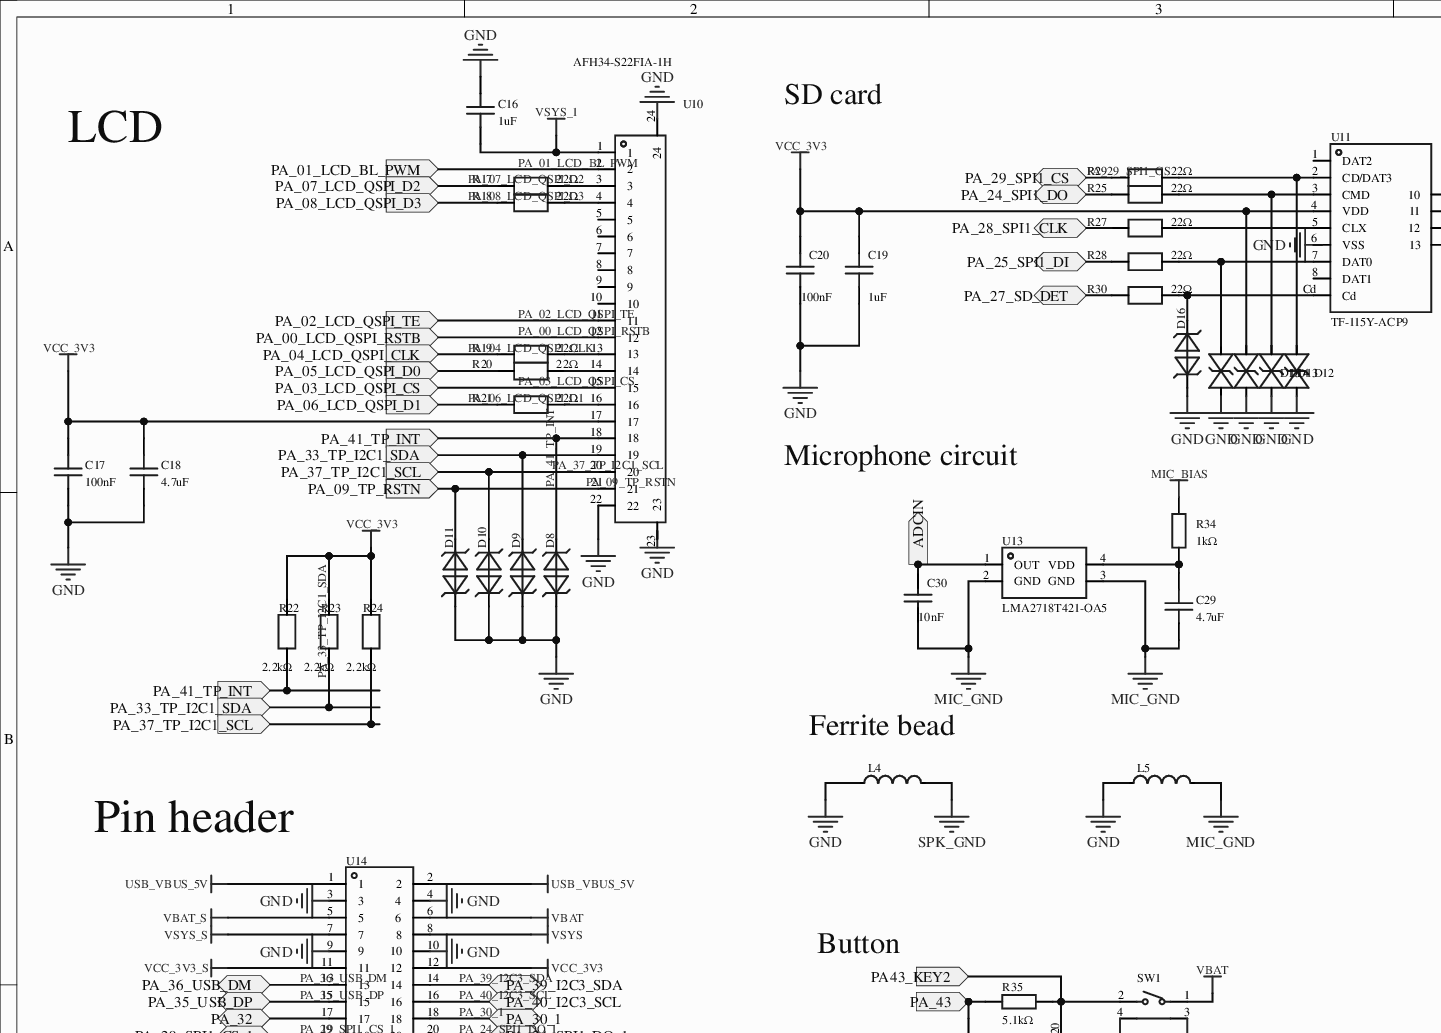
[diagram p0: MISC52032-4.schdoc, top left]
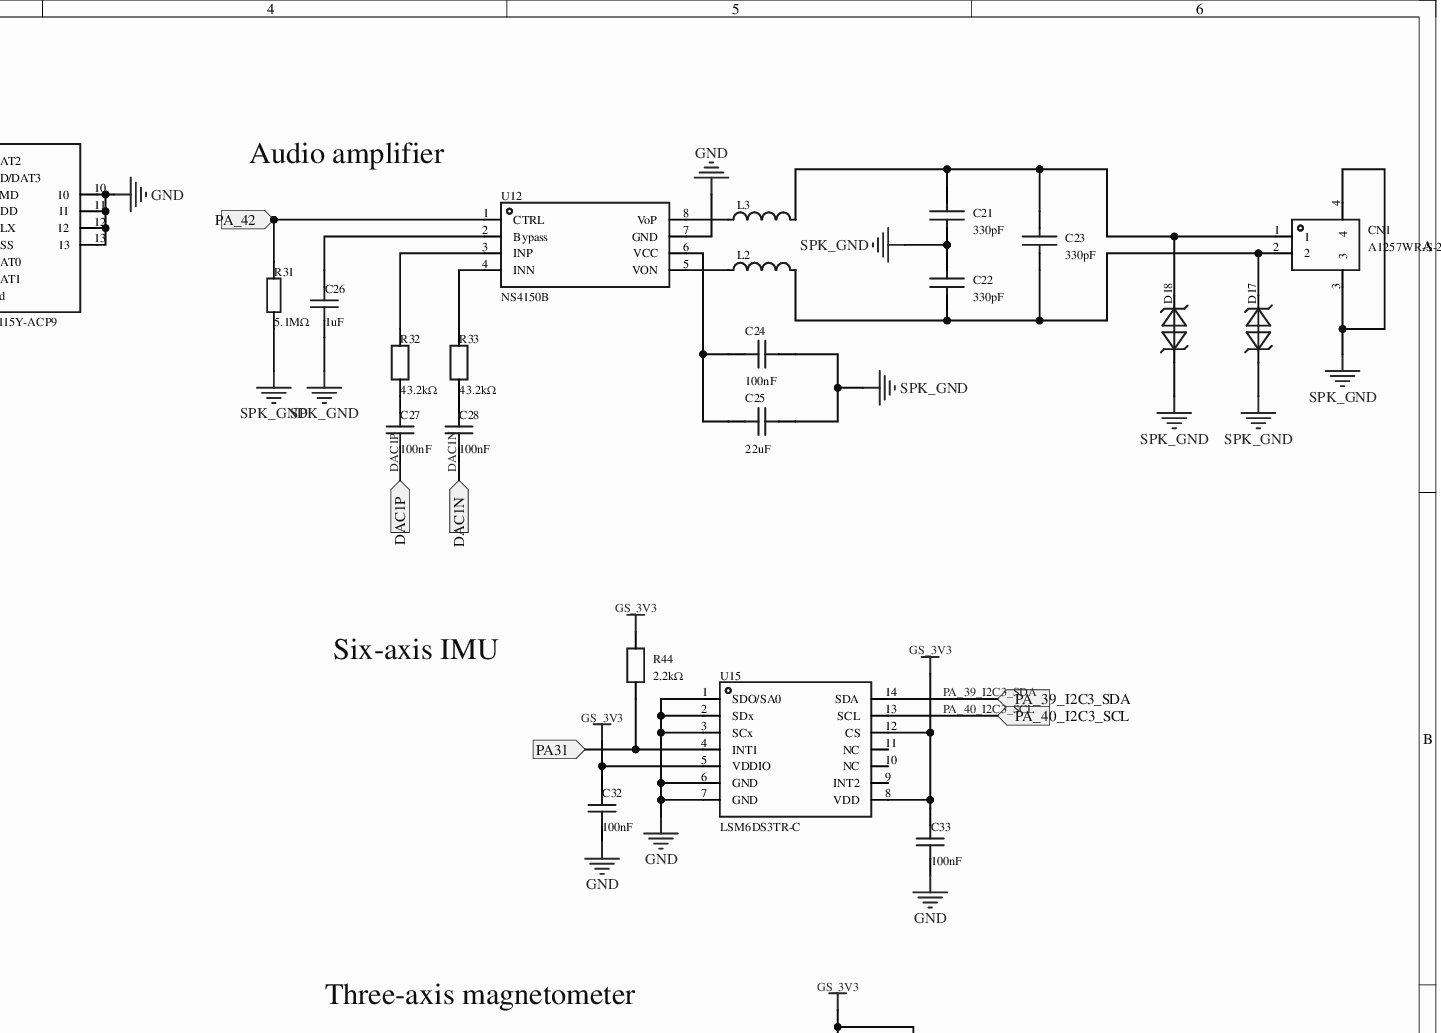
[diagram p1: MISC52032-4.schdoc, top right]
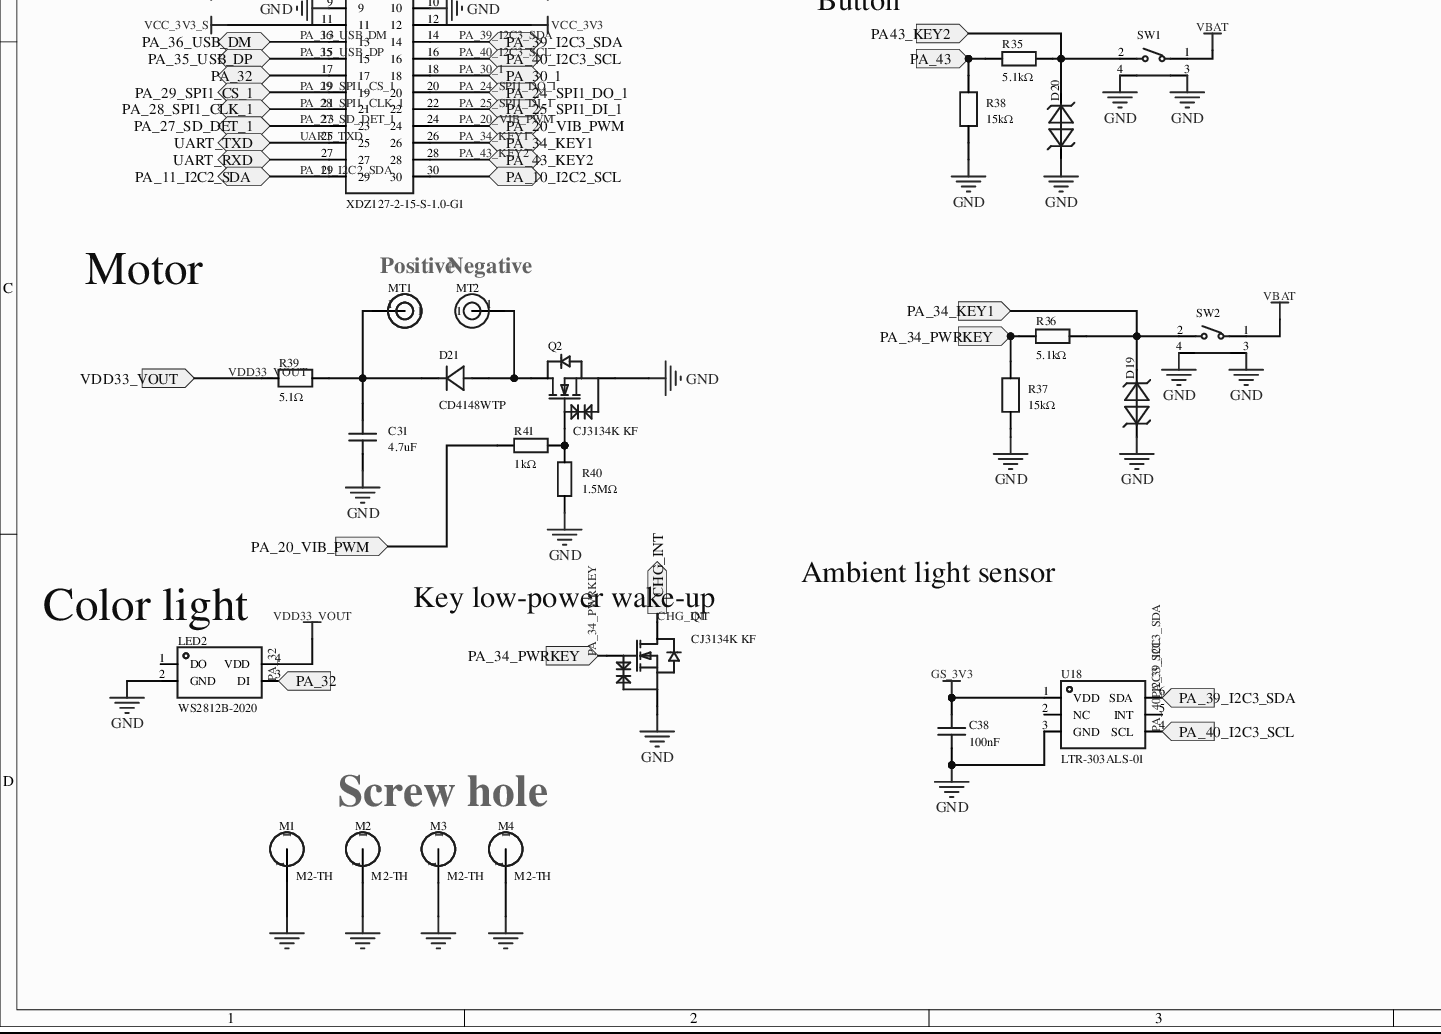
[diagram p2: MISC52032-4.schdoc, bottom left]
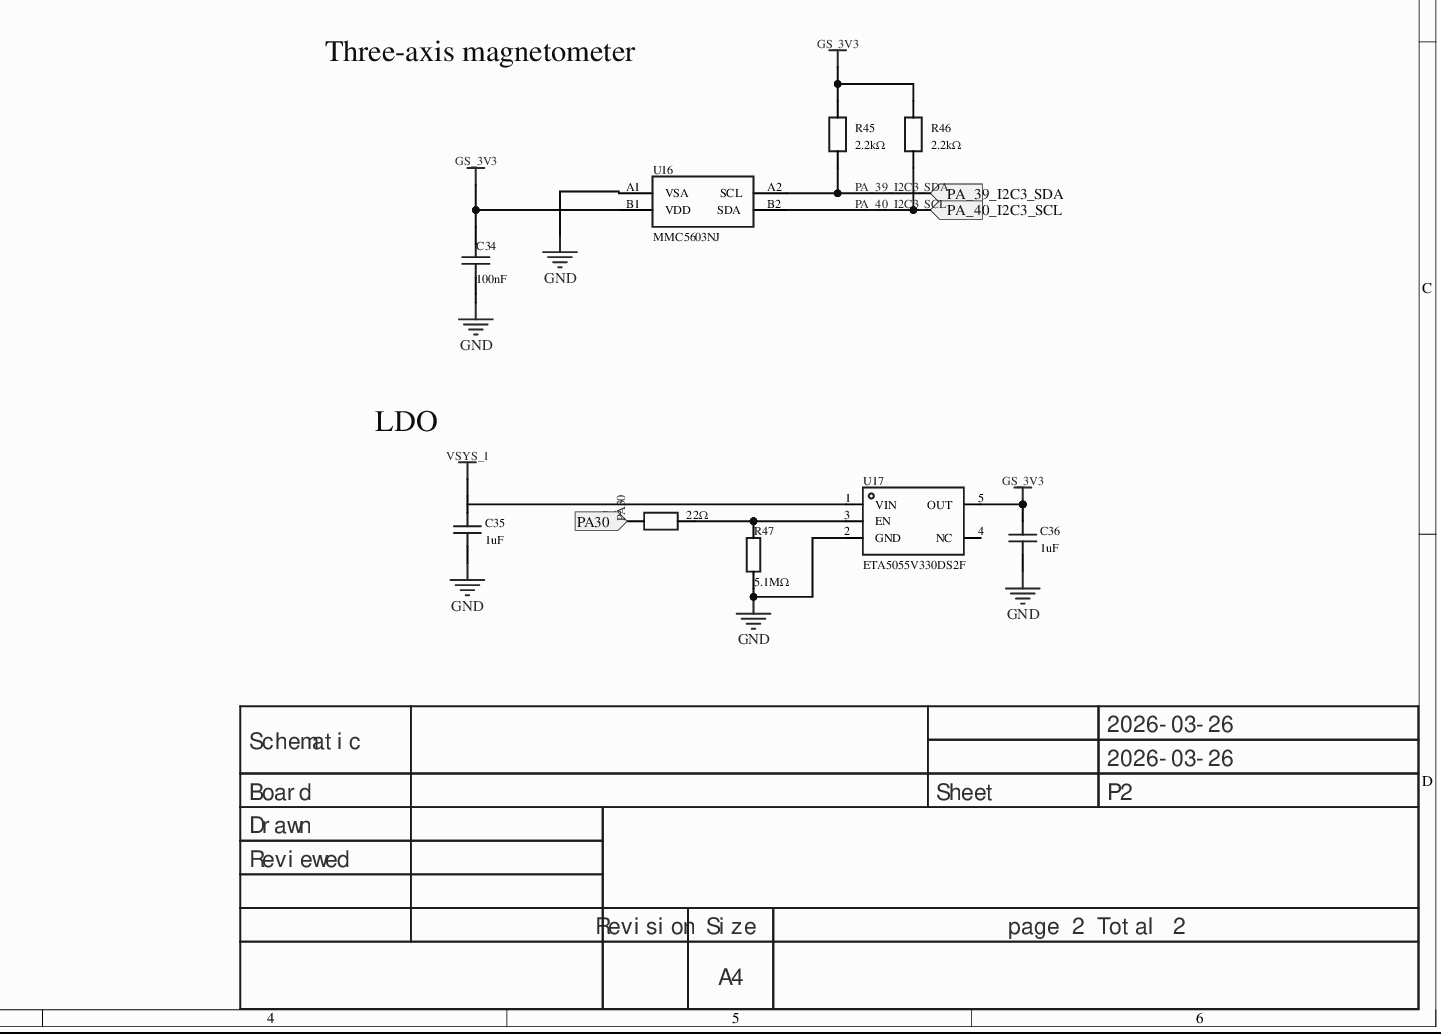
[diagram p3: MISC52032-4.schdoc, bottom right]
# Altium project MISC52032-2.PrjPcb (part 2 of 2)

## Sheet MISC52032-4.schdoc
size 420 x 297 mm; Version: V1.0; @Project Name: MISC52032; @Page Count: 2; @Update Date: 2026-03-26; @Create Date: 2026-03-26; @Schematic Name: MISC52032; @Page No: 2; @Board Name: MISC52032; @Create Time: 13:38:37; @Update Time: 21:26:46; Size: A4

### Parts
C16  1uF  [C0402]
C17  100nF  [C0402]
C18  4.7uF  [C0402]
C19  1uF  [C0402]
C20  100nF  [C0402]
C21  330pF  [C0402]
C22  330pF  [C0402]
C23  330pF  [C0402]
C24  100nF  [C0402]
C25  22uF  [C0402]
C26  1uF  [C0402]
C27  100nF  [C0402]
C28  100nF  [C0402]
C29  4.7uF  [C0402]
C30  10nF  [C0402]
C31  4.7uF  [C0402]
C32  100nF  [C0402]
C33  100nF  [C0402]
C34  100nF  [C0402]
C35  1uF  [C0402]
C36  1uF  [C0402]
C38  100nF  [C0402]
CN1  A1257WR-S-2P  [CONN-SMD_A1257WR-S-2P]
D8  ESD5451N  [DFN1006-2L-BI]  (value not drawn)
D9  ESD5451N  [DFN1006-2L-BI]  (value not drawn)
D10  ESD5451N  [DFN1006-2L-BI]  (value not drawn)
D11  ESD5451N  [DFN1006-2L-BI]  (value not drawn)
D12  (no value)  [D0402-BI]
D13  (no value)  [D0402-BI]
D14  (no value)  [D0402-BI]
D15  (no value)  [D0402-BI]
D16  ESD5451N  [DFN1006-2L-BI]  (value not drawn)
D17  ESD5451N  [DFN1006-2L-BI]  (value not drawn)
D18  ESD5451N  [DFN1006-2L-BI]  (value not drawn)
D19  ESD5451N  [DFN1006-2L-BI]  (value not drawn)
D20  ESD5451N  [DFN1006-2L-BI]  (value not drawn)
D21  CD4148WTP  [D0603-RD]
L2  (no value)  [L0402]
L3  (no value)  [L0402]
L4  (no value)  [L0603]
L5  (no value)  [L0603]
LED2  WS2812B-2020  [LED-SMD_4P-L2.0-W2.0-TL_WS2812B-2020]
M1  M2-TH  [M2_TH_4_2.5MM]
M2  M2-TH  [M2_TH_4_2.5MM]
M3  M2-TH  [M2_TH_4_2.5MM]
M4  M2-TH  [M2_TH_4_2.5MM]
MT1  (no value)  [TP-3x2MM]
MT2  (no value)  [TP-3x2MM]
Q1  CJ3134K KF  [SOT-723_L1.2-W0.8-P0.40-LS1.2-BR]
Q2  CJ3134K KF  [SOT-723_L1.2-W0.8-P0.40-LS1.2-BR]
R17  22Ω  [R0402]
R18  22Ω  [R0402]
R19  22Ω  [R0402]
R20  22Ω  [R0402]
R21  22Ω  [R0402]
R22  2.2kΩ  [R0402]
R23  2.2kΩ  [R0402]
R24  2.2kΩ  [R0402]
R25  22Ω  [R0402]
R27  22Ω  [R0402]
R28  22Ω  [R0402]
R29  22Ω  [R0402]
R30  22Ω  [R0402]
R31  5.1MΩ  [R0402]
R32  43.2kΩ  [R0402]
R33  43.2kΩ  [R0402]
R34  1kΩ  [R0402]
R35  5.1kΩ  [R0402]
R36  5.1kΩ  [R0402]
R37  15kΩ  [R0402]
R38  15kΩ  [R0402]
R39  5.1Ω  [R0402]
R40  1.5MΩ  [R0402]
R41  1kΩ  [R0402]
R44  2.2kΩ  [R0402]
R45  2.2kΩ  [R0402]
R46  2.2kΩ  [R0402]
R47  5.1MΩ  [R0402]
R48  22Ω  [R0402]
SW1  (no value)  [KEY-SMD_GT-TC191A-H026-L60]
SW2  (no value)  [KEY-SMD_GT-TC191A-H026-L60]
U10  AFH34-S22FIA-1H  [FPC-SMD_22P-P0.50_JS_AFH34-S22FIA-1H]
U11  TF-115Y-ACP9  [SIM-SMD_TF-115Y-BCP9]
U12  NS4150B  [MSOP-8_L3.0-W3.0-P0.65-LS5.0-BL]
U13  LMA2718T421-OA5  [MIC-SMD_4P-L2.8-W1.9-P1.01-TL]
U14  XDZ127-2-15-S-1.0-G1  [HDR-SMD_30P-P1.27-V-M-R2-C15-LS5.5_1]
U15  LSM6DS3TR-C  [LGA-14_L3.0-W2.5-P0.50-TL]
U16  MMC5603NJ  [FLIPCHIP-4_L0.8-W0.8-R2-C2-P0.40-TL]
U17  ETA5055V330DS2F  [SOT-23-5_L2.9-W1.6-P0.95-LS2.8-BR]
U18  LTR-303ALS-01  [TDFN-6_L2.0-W2.0-P0.65-BL]

### Ports
ADCIN (out), CHG_INT (out), DAC1N (in), DAC1P (in), PA30 (in), PA31 (in), PA43_KEY2 (in), PA_00_LCD_QSPI_RSTB (in), PA_01_LCD_BL_PWM (in), PA_02_LCD_QSPI_TE (in), PA_03_LCD_QSPI_CS (in), PA_04_LCD_QSPI_CLK (in), PA_05_LCD_QSPI_D0 (in), PA_06_LCD_QSPI_D1 (in), PA_07_LCD_QSPI_D2 (in), PA_08_LCD_QSPI_D3 (in), PA_09_TP_RSTN (in), PA_10_I2C2_SCL (bidir), PA_11_I2C2_SDA (bidir), PA_20_VIB_PWM (bidir), PA_20_VIB_PWM (in), PA_24_SPI1_DO (bidir), PA_24_SPI1_DO_1 (bidir), PA_25_SPI1_DI (bidir), PA_25_SPI1_DI_1 (bidir), PA_27_SD_DET (bidir), PA_27_SD_DET_1 (bidir), PA_28_SPI1_CLK (bidir), PA_28_SPI1_CLK_1 (bidir), PA_29_SPI1_CS (bidir), PA_29_SPI1_CS_1 (bidir), PA_30_1 (bidir), PA_32 (bidir), PA_32 (in), PA_33_TP_I2C1_SDA (in), PA_34_KEY1 (bidir), PA_34_KEY1 (in), PA_34_PWRKEY (in), PA_35_USB_DP (bidir), PA_36_USB_DM (bidir), PA_37_TP_I2C1_SCL (in), PA_39_I2C3_SDA (bidir), PA_39_I2C3_SDA (in), PA_40_I2C3_SCL (bidir), PA_40_I2C3_SCL (in), PA_41_TP_INT (in), PA_42 (in), PA_43 (in), PA_43_KEY2 (bidir), UART_RXD (bidir), UART_TXD (bidir), VDD33_VOUT (in)

### Nets
GND: C16.2 C17.1 C18.1 C19.1 C20.1 C31.1 C32.2 C33.2 C34.2 C35.1 C36.1 C38.1 D8.1 D9.1 D10.1 D11.1 D12.1(K) D13.1(K) D14.1(K) D15.1(K) D16.1 D19.1 D20.1 L4.1 L5.1 LED2.2(GND) M1.1 M2.1 M3.1 M4.1 Q1.2(S) Q2.2(S) R37.1 R38.1 R40.1 R47.1 SW1.3 SW1.4 SW2.3 SW2.4 U10.22 U10.23 U10.24 U11.6(VSS) U11.10 U11.11 U11.12 U11.13 U12.7(GND) U14.3 U14.4 U14.9 U14.10 U15.1(SDO/SA0) U15.2(SDx) U15.3(SCx) U15.6(GND) U15.7(GND) U16.A1(VSA) U17.2(GND) U18.3(GND)
GS_3V3: C32.1 C33.1 C34.1 C36.2 C38.2 R44.2 R45.2 R46.2 U15.5(VDDIO) U15.8(VDD) U15.12(CS) U16.B1(VDD) U17.5(OUT) U18.1(VDD)
MIC_BIAS: R34.2
MIC_GND: C29.1 C30.1 L5.2 U13.2(GND) U13.3(GND)
SPK_GND: C21.1 C22.2 C24.1 C25.1 C26.1 CN1.3 CN1.4 D17.1 D18.1 L4.2 R31.1
USB_VBUS_5V: U14.1 U14.2
VBAT: SW1.1 SW2.1 U14.6
VBAT_S: U14.5
VCC_3V3: C17.2 C18.2 C19.2 C20.2 D14.2(A) R22.2 R23.2 R24.2 U10.17 U11.4(VDD) U14.12
VCC_3V3_S: U14.11
VDD33_VOUT: LED2.4(VDD) R39.1 ; port VDD33_VOUT
VSYS: U14.8
VSYS_1: C16.1 C35.2 U10.1
VSYS_S: U14.7
ADCIN: C30.2 U13.1(OUT) ; port ADCIN
CHG_INT: Q1.3(D) ; port CHG_INT
DAC1N: C28.2 ; port DAC1N
DAC1P: C27.2 ; port DAC1P
PA30: R48.1 ; port PA30
PA_00_LCD_QSPI_RSTB: U10.12 ; port PA_00_LCD_QSPI_RSTB
PA_01_LCD_BL_PWM: U10.2 ; port PA_01_LCD_BL_PWM
PA_02_LCD_QSPI_TE: U10.11 ; port PA_02_LCD_QSPI_TE
PA_03_LCD_QSPI_CS: U10.15 ; port PA_03_LCD_QSPI_CS
PA_04_LCD_QSPI_CLK: R19.1 ; port PA_04_LCD_QSPI_CLK
PA_05_LCD_QSPI_D0: R20.1 ; port PA_05_LCD_QSPI_D0
PA_06_LCD_QSPI_D1: R21.1 ; port PA_06_LCD_QSPI_D1
PA_07_LCD_QSPI_D2: R17.1 ; port PA_07_LCD_QSPI_D2
PA_08_LCD_QSPI_D3: R18.1 ; port PA_08_LCD_QSPI_D3
PA_09_TP_RSTN: D11.2 U10.21 ; port PA_09_TP_RSTN
PA_10_I2C2_SCL: U14.30 ; port PA_10_I2C2_SCL
PA_11_I2C2_SDA: U14.29 ; port PA_11_I2C2_SDA
PA_20_VIB_PWM: R41.2 U14.24 ; port PA_20_VIB_PWM
PA_24_SPI1_DO_1: U14.20 ; port PA_24_SPI1_DO_1
PA_25_SPI1_DI: R28.1 ; port PA_25_SPI1_DI
PA_25_SPI1_DI_1: U14.22 ; port PA_25_SPI1_DI_1
PA_27_SD_DET: R30.1 ; port PA_27_SD_DET
PA_27_SD_DET_1: U14.23 ; port PA_27_SD_DET_1
PA_28_SPI1_CLK: R27.1 ; port PA_28_SPI1_CLK
PA_28_SPI1_CLK_1: U14.21 ; port PA_28_SPI1_CLK_1
PA_29_SPI1_CS: R29.1 ; port PA_29_SPI1_CS
PA_29_SPI1_CS_1: U14.19 ; port PA_29_SPI1_CS_1
PA_30_1: U14.18 ; port PA_30_1
PA_32: LED2.3(DI) U14.17 ; port PA_32
PA_33_TP_I2C1_SDA: D9.2 R23.1 U10.19 ; port PA_33_TP_I2C1_SDA
PA_34_KEY1: D19.2 R36.2 SW2.2 U14.26 ; port PA_34_KEY1
PA_34_PWRKEY: Q1.1(G) R36.1 R37.2 ; port PA_34_PWRKEY
PA_35_USB_DP: U14.15 ; port PA_35_USB_DP
PA_36_USB_DM: U14.13 ; port PA_36_USB_DM
PA_37_TP_I2C1_SCL: D10.2 R24.1 U10.20 ; port PA_37_TP_I2C1_SCL
PA_39_I2C3_SDA: R45.1 U14.14 U15.14(SDA) U16.A2(SCL) U18.6(SDA) ; port PA_39_I2C3_SDA
PA_40_I2C3_SCL: R46.1 U14.16 U15.13(SCL) U16.B2(SDA) U18.4(SCL) ; port PA_40_I2C3_SCL
PA_41_TP_INT: D8.2 R22.1 U10.18 ; port PA_41_TP_INT
PA_42: R31.2 U12.1(CTRL) ; port PA_42
PA_43: R35.1 R38.2 ; port PA_43
PA_43_KEY2: U14.28 ; port PA_43_KEY2
UART_RXD: U14.27 ; port UART_RXD
UART_TXD: U14.25 ; port UART_TXD
NetC21_2: C21.2 C23.2 CN1.1 D18.2 L3.2
NetC22_1: C22.1 C23.1 CN1.2 D17.2 L2.2
NetC24_2: C24.2 C25.2 U12.6(VCC)
NetC26_2: C26.2 U12.2(Bypass)
NetC27_1: C27.1 R32.1
NetC28_1: C28.1 R33.1
NetC29_2: C29.2 R34.1 U13.4(VDD)
NetC31_2: C31.2 D21.1(K) MT1.1 R39.2
NetD12_2: D12.2(A) R29.2 U11.2(CD/DAT3)
NetD13_2: D13.2(A) R25.2 U11.3(CMD)
NetD15_2: D15.2(A) R28.2 U11.7(DAT0)
NetD16_2: D16.2 R30.2 U11.Cd
NetD20_2: D20.2 R35.2 SW1.2 ; port PA43_KEY2
NetD21_2: D21.2(A) MT2.1 Q2.3(D)
NetL2_1: L2.1 U12.5(VON)
NetL3_1: L3.1 U12.8(VoP)
NetQ2_1: Q2.1(G) R40.2 R41.1
NetR17_2: R17.2 U10.3
NetR18_2: R18.2 U10.4
NetR19_2: R19.2 U10.13
NetR20_2: R20.2 U10.14
NetR21_2: R21.2 U10.16
NetR25_1: R25.1 ; port PA_24_SPI1_DO
NetR27_2: R27.2 U11.5(CLX)
NetR32_2: R32.2 U12.3(INP)
NetR33_2: R33.2 U12.4(INN)
NetR44_1: R44.1 U15.4(INT1) ; port PA31
NetR47_2: R47.2 R48.2 U17.3(EN)

Not connected (* = marked no-connect by the designer): LED2 1(DO)*; U10 5* 6* 7* 8* 9* 10*; U11 1(DAT2)* 8(DAT1)*; U15 9(INT2)* 10(NC)* 11(NC)*; U17 1(VIN) 4(NC)*; U18 2(NC)* 5(INT)*

### Notes on the sheet
- LCD
- SD card
- (near U12) Audio amplifier
- Microphone circuit
- Six-axis IMU
- (near L4) Ferrite bead
- (near U14) Pin header
- Button
- Three-axis magnetometer
- Motor
- Positive
- Negative
- LDO
- (near LED2) Color light
- (near Q1) Key low-power wake-up
- Ambient light sensor
- Screw hole
- 2026-03-26
- Schematic
- Board
- Sheet
- P2
- Drawn
- Reviewed
- Revision
- Size
- A4
- page 2 Total 2

### Library data of the parts
C16 C19 C26 C35 C36 = CL05A105KA5NQNC: Capacitance:1uF;Tolerance:±10%;Rated voltage:25V;Temperature coefficient:X5R;; Manufacturer: SAMSUNG(三星); AddInBom: yes; ModelId: 36a51122f27c49738f86b3bfa98863e0; ModelName: C0402_L1.0-W0.5-H0.5; ModelTransform: 39.37,19.685,0,0,0,0,0,0,0; Tolerance: ±10%; Voltage Rating: 25V; Temperature Coefficient: X5R; Symbol: CL05A105KA5NQNC; Device: CL05A105KA5NQNC; LCSC Part Name: 1uF ±10% 25V; SupplierPart: C52923; ManufacturerPart: CL05A105KA5NQNC; Supplier Footprint: 0402; JLCPCB Part Class: Basic library; Datasheet: example.com/datasheet/CL05A105KA5NQNC/53938.html; Supplier: LCSC; ConvertToPcb: yes; FootprintName: C0402; Value: 1uF
C17 C20 C24 C27 C28 C32-C34 C38 = CL05B104KO5NNNC: Capacitance:100nF;Tolerance:±10%;Rated voltage:16V;Temperature coefficient:X7R;; Manufacturer: SAMSUNG(三星); AddInBom: yes; ModelId: 36a51122f27c49738f86b3bfa98863e0; ModelName: C0402_L1.0-W0.5-H0.5; ModelTransform: 39.37,19.685,0,0,0,0,0,0,0; Tolerance: ±10%; Voltage Rating: 16V; Temperature Coefficient: X7R; Symbol: CL05B104KO5NNNC; Device: CL05B104KO5NNNC; LCSC Part Name: 100nF ±10% 16V; SupplierPart: C1525; ManufacturerPart: CL05B104KO5NNNC; Supplier Footprint: 0402; JLCPCB Part Class: Basic library; Datasheet: example.com/datasheet/CL05B104KO5NNNC/1877.html; Supplier: LCSC; ConvertToPcb: yes; FootprintName: C0402; Value: 100nF
C18 C29 C31 = CL05A475MP5NRNC: Capacitance:4.7uF;Tolerance:±20%;Rated voltage:10V;Temperature coefficient:X5R;; Manufacturer: SAMSUNG(三星); AddInBom: yes; ModelId: 36a51122f27c49738f86b3bfa98863e0; ModelName: C0402_L1.0-W0.5-H0.5; ModelTransform: 39.37,19.685,0,0,0,0,0,0,0; Tolerance: ±20%; Voltage Rating: 10V; Temperature Coefficient: X5R; Symbol: CL05A475MP5NRNC; Device: CL05A475MP5NRNC; LCSC Part Name: 4.7uF ±20% 10V; SupplierPart: C23733; ManufacturerPart: CL05A475MP5NRNC; Supplier Footprint: 0402; JLCPCB Part Class: Basic library; Datasheet: example.com/datasheet/CL05A475MP5NRNC/24469.html; Supplier: LCSC; ConvertToPcb: yes; FootprintName: C0402; Value: 4.7uF
C21-C23 = CL05C331JB5NNNC: Capacitance:330pF;Tolerance:±5%;Rated voltage:50V;Temperature coefficient:C0G;; Manufacturer: SAMSUNG(三星); AddInBom: yes; ModelId: 36a51122f27c49738f86b3bfa98863e0; ModelName: C0402_L1.0-W0.5-H0.5; ModelTransform: 39.37,19.685,0,0,0,0,0,0,0; Tolerance: ±5%; Voltage Rating: 50V; Temperature Coefficient: C0G; Symbol: CL05C331JB5NNNC; Device: CL05C331JB5NNNC; LCSC Part Name: 330pF ±5% 50V; SupplierPart: C13533; ManufacturerPart: CL05C331JB5NNNC; Supplier Footprint: 0402; JLCPCB Part Class: Extended library; Datasheet: example.com/datasheet/CL05C331JB5NNNC/14182.html; Supplier: LCSC; ConvertToPcb: yes; FootprintName: C0402; Value: 330pF
C25 = GRM155R60J226ME11D: Capacitance:22uF;Tolerance:±20%;Rated voltage:6.3V;Temperature coefficient:X5R;; Manufacturer: muRata(村田); AddInBom: yes; ModelId: 36a51122f27c49738f86b3bfa98863e0; ModelName: C0402_L1.0-W0.5-H0.5; ModelTransform: 39.37,19.685,0,0,0,0,0,0,0; Tolerance: ±20%; Voltage Rating: 6.3V; Temperature Coefficient: X5R; Symbol: GRM155R60J226ME11D; Device: GRM155R60J226ME11D; LCSC Part Name: 22uF ±20% 6.3V; SupplierPart: C415703; ManufacturerPart: GRM155R60J226ME11D; Supplier Footprint: 0402; JLCPCB Part Class: Extended library; Datasheet: example.com/datasheet/GRM155R60J226ME11D/408393.html; Supplier: LCSC; ConvertToPcb: yes; FootprintName: C0402; Value: 22uF
C30 = CL05B103KB5NNNC: Capacitance:10nF;Tolerance:±10%;Rated voltage:50V;Temperature coefficient:X7R;; Manufacturer: SAMSUNG(三星); AddInBom: yes; ModelId: 36a51122f27c49738f86b3bfa98863e0; ModelName: C0402_L1.0-W0.5-H0.5; ModelTransform: 39.37,19.685,0,0,0,0,0,0,0; Tolerance: ±10%; Voltage Rating: 50V; Temperature Coefficient: X7R; Symbol: CL05B103KB5NNNC; Device: CL05B103KB5NNNC; LCSC Part Name: 10nF ±10% 50V; SupplierPart: C15195; ManufacturerPart: CL05B103KB5NNNC; Supplier Footprint: 0402; JLCPCB Part Class: Basic library; Datasheet: example.com/datasheet/CL05B103KB5NNNC/15869.html; Supplier: LCSC; ConvertToPcb: yes; FootprintName: C0402; Value: 10nF
CN1 = A1257WR-S-2P: Pin structure:1x2P;Pitch:1.25mm;Mounting:Horizontal;Reference series:GH;Total pins:2P;Rows:1;Pins per row:2;Row spacing:-;Rated current:1A;Contact material:Phosphor bronze;Contact plating:Tin;Operating temperature:-40℃~+105℃;; Manufacturer: CJT(长江连接器); AddInBom: yes; ModelId: dbecf4c343244a1e903fd8658ee1ce26; ModelName: CONN-SMD_GH1.25-WS-2P; ModelTransform: 226.378,191.3382,0,0,0,0,0,-16.811,0; Pins Structure: 1x2P; Pitch: 1.25mm; Reference Series: GH; Number of PINs Per Row: 2; Current Rating: 1A; Voltage Rating: 50V; Plastic Material: PA9T; Flame Retardant Rating: UL94V-0; Symbol: A1257WR-S-2P; Device: A1257WR-S-2P; LCSC Part Name: 1x2P 间距:1.25mm 卧贴 系列:GH; SupplierPart: C225125; ManufacturerPart: A1257WR-S-2P; Supplier Footprint: SMD,P=1.25mm,卧贴; JLCPCB Part Class: Extended library; Datasheet: example.com/datasheet/A1257WR-S-2P/225408.html; Supplier: LCSC; ConvertToPcb: yes; FootprintName: CONN-SMD_A1257WR-S-2P; Mounting Type: Horizontal mount; Number of Pins: 2P; Number of Rows: 1; Row Spacing: -; Contact Material: Phosphor bronze; Contact Plating: Tin; Operating Temperature: -40℃~+105℃; Color: -
D8-D11 D16-D20 = ESD5451N: Manufacturer: UMW(友台半导体); 3D Model: 2bdbcca3b35b49c5a8ae725a08658930; Type: ESD; AddInBom: yes; ModelTransform: 40.1574,24.4094,0,0,0,0,0,0,0; Supplier Footprint: DFN1006-2; JLCPCB Part Class: Extended Part; Datasheet: example.com/upload/public/pdf/source/20231109/ADF50DFDA976AEDE26D2560D9AE1EB02.pdf; Device: ESD5451N; Symbol: ESD5451N; LCSC Part Name: ESD5451N; SupplierPart: C2987696; ManufacturerPart: ESD5451N; Supplier: LCSC; ConvertToPcb: yes; FootprintName: DFN1006-2L-BI; ModelName: DFN1006-2L-BI
D12-D15 = KLXES15AAA1: Polarity:Bidirectional;Reverse standoff voltage (Vrwm):5V;Clamping voltage:40V;Peak pulse current (Ipp):-;Peak pulse power (Ppp):-;Breakdown voltage:-;; Manufacturer: KUU; AddInBom: yes; ModelId: 62a80a189f1b46df8ba79817b730b378; ModelName: D0402_L1.0-W0.5-H0.5; ModelTransform: 39.37,19.685,0,0,0,0,0,0,0; Reverse Stand-Off Voltage (Vrwm): 5V; Clamping Voltage: 40V; Reverse Leakage Current (Ir): 10nA; Number of Channels: Single channel; level of protection: IEC 61000-4-2; Type: ESD; Junction Capacitance: 0.05pF; Symbol: KLXES15AAA1; Device: KLXES15AAA1; LCSC Part Name: 双向ESD 5V截止; SupplierPart: C2892490; Supplier Footprint: 0402; JLCPCB Part Class: Extended library; Datasheet: example.com/datasheet/KLXES15AAA1/3124109.html; Supplier: LCSC; ConvertToPcb: yes; FootprintName: D0402-BI; Polarity: Bidirectional; Peak Pulse Current (Ipp): -; Peak Pulse Power Dissipation (Ppp): -; Voltage - Breakdown: -; Operating Temperature: -55℃~+125℃
D21 = CD4148WTP_C30584800: Diode configuration:Discrete;Forward voltage (Vf):1.25V@100mA;DC reverse voltage (Vr):75V;Rectified current:150mA;Reverse recovery time (Trr):4ns;; Manufacturer: YONGYUTAI(永裕泰); AddInBom: yes; ModelId: 35f9a12e738d4b13b3012a5e6f6e8360; ModelTransform: 61.024,31.496,0,0,0,0,0,0,0; Voltage - DC Reverse(Vr): 75V; Current - Rectified: 150mA; Pd - Power Dissipation: 200mW; Reverse Leakage Current (Ir): 5uA@75V; Reverse Recovery Time (trr): 4ns; Operating Junction Temperature Range: -55℃~+150℃@(Tj); Non-Repetitive Peak Forward Surge Current: 800mA; Symbol: CD4148WTP_C30584800; Device: CD4148WTP_C30584800; LCSC Part Name: 75V 150mA; SupplierPart: C30584800; ManufacturerPart: CD4148WTP; Supplier Footprint: 0603; JLCPCB Part Class: Extended library; Datasheet: example.com/datasheet/CD4148WTP/32319012.html; Supplier: LCSC; ConvertToPcb: yes; FootprintName: D0603-RD; ModelName: D0603-RD; Diode Configuration: Discrete; Voltage - Forward(Vf@If): 1.25V@100mA
L2 L3 = PZ1005U121-1R0TF: Impedance@frequency:120Ω@100MHz;Tolerance:±25%;DC resistance (DCR):120mΩ;; Manufacturer: Sunlord(顺络); AddInBom: yes; ModelId: d8d36575a3234d4790bfa765c88664a7; ModelName: L0402_L1.0-W0.5-H0.5_BEAD; ModelTransform: 39.37,19.685,0,0,0,0,0,0.0005,0; Tolerance: ±25%; DC Resistance(DCR): 120mΩ; Current Rating: 1A; Number of Circuits: 1; Symbol: PZ1005U121-1R0TF; Device: PZ1005U121-1R0TF; LCSC Part Name: 单路 0402磁珠 阻抗120Ω@100MHz; SupplierPart: C96723; Supplier Footprint: 0402; JLCPCB Part Class: Extended library; Datasheet: example.com/datasheet/PZ1005U121-1R0TF/97928.html; Supplier: LCSC; ConvertToPcb: yes; FootprintName: L0402; Impedance @ Frequency: 120Ω@100MHz
L4 L5 = CBG160808U000T: Impedance@frequency:0Ω@100MHz;DC resistance (DCR):100mΩ;; Manufacturer: FH(风华); AddInBom: yes; ModelId: 2bc5ec593d464d6ba9807aec0b5673c2; ModelName: L0603_L1.6-W0.8-H0.5_BEAD; ModelTransform: 62.992,31.496,0,180,0,0,0.094,0.629,0; DC Resistance(DCR): 100mΩ; Current Rating: 800mA; Number of Circuits: 1; Symbol: CBG160808U000T; Device: CBG160808U000T; LCSC Part Name: 单路 0603磁珠 阻抗0Ω@100MHz; SupplierPart: C43163; Supplier Footprint: 0603; JLCPCB Part Class: Extended library; Datasheet: example.com/datasheet/CBG160808U000T/44154.html; Supplier: LCSC; ConvertToPcb: yes; FootprintName: L0603; Impedance @ Frequency: 0Ω@100MHz; Operating Temperature: -40℃~+85℃
LED2 = WS2812B-2020: 12mA, small size, high brightness, for small-pitch small-size products (note moisture sensitivity; see datasheet for details); Manufacturer: worldsemi; AddInBom: yes; ModelId: ec3f1773c2c342958c28fcec35b8a247; ModelName: LED-SMD_4P-L2.0-W2.0-H0.8-TL_WS2812B-2020; ModelTransform: 78.74,78.74,0,0,0,0,0.001,0.005,0; Wavelength: 515.6nm; 622.5nm; 470.4nm; Luminous Intensity: 200mcd; 160mcd; 520mcd; Data Transmission Rate: 100KB/S; Voltage - Supply: 5V; Installation method: Top mount; Symbol: WS2812B-2020; Device: WS2812B-2020; LCSC Part Name: RGB三色; SupplierPart: C965555; ManufacturerPart: WS2812B-2020; Supplier Footprint: SMD,2.2x2mm; JLCPCB Part Class: Extended library; Datasheet: example.com/datasheet/WS2812B-2020/1051115.html; Supplier: LCSC; ConvertToPcb: yes; FootprintName: LED-SMD_4P-L2.0-W2.0-TL_WS2812B-2020; Fixed-Frequency Pwm Mode: -; Quiescent Current: -; Lens Color: -; ESD Withstand Voltage: -; Operating Temperature: -
M1-M4 = M2-TH: Check: false; AddInBom: no; ConvertToPcb: yes; Device: M2-TH; SymbolName: M2-TH; FootprintName: M2_TH_4_2.5MM; Value: M2-TH
MT1 MT2 = TP_2x3MM: Add into BOM: no; Check: false; ConvertToPcb: yes; SymbolName: TP; Device: TP_2x3MM; FootprintName: TP-3x2MM
Q1 Q2 = CJ3134K KF: Type:1 N-channel;Drain-source voltage (Vdss):20V;Continuous drain current (Id):750mA;On-resistance (RDS(on)):380mΩ@4.5V,650mA;Power dissipation (Pd):150mW;Threshold voltage (Vgs(th)):1.1V;; Manufacturer: CJ(江苏长电/长晶); Symbol: CJ3134K_C62503; AddInBom: yes; ModelId: abccde1e67074d7481274a37cf5c97f0; ModelName: SOT-723-3P_L1.2-W0.8-H0.6-LS1.2-P0.40; ModelTransform: 47.244,47.244,0,180,0,0,0,0,0; Drain to Source Voltage: 20V; Current - Continuous Drain(Id): 750mA; Pd - Power Dissipation: 150mW; Gate Threshold Voltage (Vgs(th)@Id): 1.1V; Device: CJ3134K KF; LCSC Part Name: 1个N沟道 耐压:20V 电流:750mA; SupplierPart: C62503; ManufacturerPart: CJ3134K KF; Supplier Footprint: SOT-723; JLCPCB Part Class: Extended library; Datasheet: example.com/upload/public/pdf/source/20160416/1460799387864.pdf; Supplier: LCSC; ConvertToPcb: yes; FootprintName: SOT-723_L1.2-W0.8-P0.40-LS1.2-BR; Type: 1 N-channel; RDS(on): 380mΩ@4.5V,650mA
R17-R21 R25 R27-R30 R48 = FRC0402J220 TS: Resistor type:Thick-film resistor;Resistance:22Ω;Tolerance:±5%;Power:62.5mW;Operating voltage:50V;Temperature coefficient:±100ppm/℃;; Manufacturer: FOJAN(富捷); AddInBom: yes; ModelId: 98c88bc2b9094f218f3a3e30a7012738; ModelName: R0402_L1.0-W0.5-H0.4; ModelTransform: 39.37,19.685,0,0,0,0,0,0,0; Tolerance: ±5%; Power(Watts): 62.5mW; Voltage-Supply(Max): 50V; Symbol: FRC0402J220 TS; Device: FRC0402J220 TS; LCSC Part Name: 22Ω ±5% 62.5mW 厚膜电阻; SupplierPart: C2906914; ManufacturerPart: FRC0402J220 TS; Supplier Footprint: 0402; JLCPCB Part Class: Extended library; Datasheet: example.com/datasheet/FRC0402J220%2520TS/3180427.html; Supplier: LCSC; ConvertToPcb: yes; FootprintName: R0402; Type: Thick-film resistor; Value: 22Ω; Temperature Coefficient: ±100ppm/℃; Operating Temperature: -55℃~+155℃
R22-R24 R44-R46 = FRC0402F2201TS: Resistor type:Thick-film resistor;Resistance:2.2kΩ;Tolerance:±1%;Power:62.5mW;Operating voltage:50V;Temperature coefficient:±100ppm/℃;; Manufacturer: FOJAN(富捷); AddInBom: yes; ModelId: 98c88bc2b9094f218f3a3e30a7012738; ModelName: R0402_L1.0-W0.5-H0.4; ModelTransform: 39.37,19.685,0,0,0,0,0,0,0; Tolerance: ±1%; Power(Watts): 62.5mW; Voltage-Supply(Max): 50V; Symbol: FRC0402F2201TS; Device: FRC0402F2201TS; LCSC Part Name: 2.2kΩ ±1% 62.5mW 厚膜电阻; SupplierPart: C2906865; ManufacturerPart: FRC0402F2201TS; Supplier Footprint: 0402; JLCPCB Part Class: Extended library; Datasheet: example.com/datasheet/FRC0402F2201TS/3180378.html; Supplier: LCSC; ConvertToPcb: yes; FootprintName: R0402; Type: Thick-film resistor; Value: 2.2kΩ; Temperature Coefficient: ±100ppm/℃; Operating Temperature: -55℃~+155℃
R31 R47 = 0402WGF5104TCE: Resistor type:Thick-film resistor;Resistance:5.1MΩ;Tolerance:±1%;Power:62.5mW;Operating voltage:50V;Temperature coefficient:±100ppm/℃;; Manufacturer: UNI-ROYAL(厚声); AddInBom: yes; ModelId: 98c88bc2b9094f218f3a3e30a7012738; ModelName: R0402_L1.0-W0.5-H0.4; ModelTransform: 39.37,19.685,0,0,0,0,0,0,0; Tolerance: ±1%; Power(Watts): 62.5mW; Voltage-Supply(Max): 50V; Symbol: 0402WGF5104TCE; Device: 0402WGF5104TCE; LCSC Part Name: 5.1MΩ ±1% 62.5mW 厚膜电阻; SupplierPart: C270595; ManufacturerPart: 0402WGF5104TCE; Supplier Footprint: 0402; JLCPCB Part Class: Extended library; Datasheet: example.com/datasheet/0402WGF5104TCE/259975.html; Supplier: LCSC; ConvertToPcb: yes; FootprintName: R0402; Type: Thick-film resistor; Value: 5.1MΩ; Temperature Coefficient: ±100ppm/℃; Operating Temperature: -55℃~+155℃
R32 R33 = FRC0402F4322TS: Resistor type:Thick-film resistor;Resistance:43.2kΩ;Tolerance:±1%;Power:62.5mW;Operating voltage:50V;Temperature coefficient:±100ppm/℃;; Manufacturer: FOJAN(富捷); AddInBom: yes; ModelId: 98c88bc2b9094f218f3a3e30a7012738; ModelName: R0402_L1.0-W0.5-H0.4; ModelTransform: 39.37,19.685,0,0,0,0,0,0,0; Tolerance: ±1%; Power(Watts): 62.5mW; Voltage-Supply(Max): 50V; Symbol: FRC0402F4322TS; Device: FRC0402F4322TS; LCSC Part Name: 43.2kΩ ±1% 62.5mW 厚膜电阻; SupplierPart: C2906870; ManufacturerPart: FRC0402F4322TS; Supplier Footprint: 0402; JLCPCB Part Class: Extended library; Supplier: LCSC; ConvertToPcb: yes; FootprintName: R0402; Type: Thick-film resistor; Value: 43.2kΩ; Temperature Coefficient: ±100ppm/℃; Operating Temperature: -55℃~+155℃
R34 R41 = RC0402FR-071KL: Resistor type:Thick-film resistor;Resistance:1kΩ;Tolerance:±1%;Power:62.5mW;Operating voltage:50V;Temperature coefficient:±100ppm/℃;; Manufacturer: YAGEO(国巨); AddInBom: yes; ModelId: 98c88bc2b9094f218f3a3e30a7012738; ModelName: R0402_L1.0-W0.5-H0.4; ModelTransform: 39.37,19.685,0,0,0,0,0,0,0; Tolerance: ±1%; Power(Watts): 62.5mW; Voltage-Supply(Max): 50V; Symbol: RC0402FR-071KL; Device: RC0402FR-071KL; LCSC Part Name: 厚膜电阻 1kΩ ±1% 62.5mW; SupplierPart: C106235; ManufacturerPart: RC0402FR-071KL; Supplier Footprint: 0402; JLCPCB Part Class: Extended library; Datasheet: example.com/datasheet/RC0402FR-071KL/107450.html; Supplier: LCSC; ConvertToPcb: yes; FootprintName: R0402; Type: Thick-film resistor; Value: 1kΩ; Temperature Coefficient: ±100ppm/℃; Operating Temperature: -55℃~+155℃
R35 R36 = 0402WGF5101TCE: Resistor type:Thick-film resistor;Resistance:5.1kΩ;Tolerance:±1%;Power:62.5mW;Operating voltage:50V;Temperature coefficient:±100ppm/℃;; Manufacturer: UNI-ROYAL(厚声); AddInBom: yes; ModelId: 98c88bc2b9094f218f3a3e30a7012738; ModelName: R0402_L1.0-W0.5-H0.4; ModelTransform: 39.37,19.685,0,0,0,0,0,0,0; Tolerance: ±1%; Power(Watts): 62.5mW; Voltage-Supply(Max): 50V; Symbol: 0402WGF5101TCE; Device: 0402WGF5101TCE; LCSC Part Name: 5.1kΩ ±1% 62.5mW 厚膜电阻; SupplierPart: C25905; ManufacturerPart: 0402WGF5101TCE; Supplier Footprint: 0402; JLCPCB Part Class: Basic library; Datasheet: example.com/datasheet/0402WGF5101TCE/26648.html; Supplier: LCSC; ConvertToPcb: yes; FootprintName: R0402; Type: Thick-film resistor; Value: 5.1kΩ; Temperature Coefficient: ±100ppm/℃; Operating Temperature: -55℃~+155℃
R37 R38 = FRC0402F1502TS: Resistor type:Thick-film resistor;Resistance:15kΩ;Tolerance:±1%;Power:62.5mW;Operating voltage:50V;Temperature coefficient:±100ppm/℃;; Manufacturer: FOJAN(富捷); AddInBom: yes; ModelId: 98c88bc2b9094f218f3a3e30a7012738; ModelName: R0402_L1.0-W0.5-H0.4; ModelTransform: 39.37,19.685,0,0,0,0,0,0,0; Tolerance: ±1%; Power(Watts): 62.5mW; Voltage-Supply(Max): 50V; Symbol: FRC0402F1502TS; Device: FRC0402F1502TS; LCSC Part Name: 15kΩ ±1% 62.5mW 厚膜电阻; SupplierPart: C2909322; ManufacturerPart: FRC0402F1502TS; Supplier Footprint: 0402; JLCPCB Part Class: Extended library; Supplier: LCSC; ConvertToPcb: yes; FootprintName: R0402; Type: Thick-film resistor; Value: 15kΩ; Temperature Coefficient: ±100ppm/℃; Operating Temperature: -55℃~+155℃
R39 = FRC0402F5R10TS: Resistor type:Thick-film resistor;Resistance:5.1Ω;Tolerance:±1%;Power:62.5mW;Operating voltage:50V;Temperature coefficient:±200ppm/℃;; Manufacturer: FOJAN(富捷); AddInBom: yes; ModelId: 98c88bc2b9094f218f3a3e30a7012738; ModelName: R0402_L1.0-W0.5-H0.4; ModelTransform: 39.37,19.685,0,0,0,0,0,0,0; Tolerance: ±1%; Power(Watts): 62.5mW; Voltage-Supply(Max): 50V; Symbol: FRC0402F5R10TS; Device: FRC0402F5R10TS; LCSC Part Name: 5.1Ω ±1% 62.5mW 厚膜电阻; SupplierPart: C2909363; ManufacturerPart: FRC0402F5R10TS; Supplier Footprint: 0402; JLCPCB Part Class: Extended library; Datasheet: example.com/datasheet/FRC0402F5R10TS/3186298.html; Supplier: LCSC; ConvertToPcb: yes; FootprintName: R0402; Type: Thick-film resistor; Value: 5.1Ω; Temperature Coefficient: ±200ppm/℃; Operating Temperature: -55℃~+155℃
R40 = RCT021M5JLF: Resistance:1.5MΩ;Tolerance:±5%;Power:62.5mW;; Manufacturer: HKR(香港电阻); AddInBom: yes; ModelId: 98c88bc2b9094f218f3a3e30a7012738; ModelName: R0402_L1.0-W0.5-H0.4; ModelTransform: 39.37,19.685,0,0,0,0,0,0,0; Tolerance: ±5%; Power(Watts): 62.5mW; Symbol: RCT021M5JLF; Device: RCT021M5JLF; LCSC Part Name: 1.5MΩ ±5% 62.5mW; SupplierPart: C174197; ManufacturerPart: RCT021M5JLF; Supplier Footprint: 0402; JLCPCB Part Class: Extended library; Datasheet: example.com/upload/public/pdf/source/20180327/C185769_D03C9885E3618D1189E898A32FE91026.pdf; Supplier: LCSC; ConvertToPcb: yes; FootprintName: R0402; Value: 1.5MΩ
SW1 SW2 = GT-TC191A-H026-L60: Circuit structure:SPST;Button shape:Round button;Actuation force:1.8N;Mounting:Horizontal;Switch length:4.5mm;Switch width:2.2mm;Switch height:2.6mm;Bracket:Without bracket;Contact current:50mA;Rated voltage:12V;Lamp:None;Operating life:600万 cycles;; Manufacturer: G-Switch(品赞); AddInBom: yes; ModelId: feac9e81515c4f30b5bbf11a83781aa2; ModelTransform: 177.165,118.11,0,0,0,0,0,-33.425,-23.622; Circuit: SPST; Operating Force: 1.8N; Switch Height: 2.6mm; Contact Current: 50mA; Voltage Rating: 12V; Actuator/Cap Color: Black; With Lamp: None; Symbol: GT-TC191A-H026-L60; Device: GT-TC191A-H026-L60; LCSC Part Name: 2.2*4.5*2.6mm 卧贴 轻触开关; SupplierPart: C2890363; Supplier Footprint: SMD,4.5x2.2mm; JLCPCB Part Class: Extended library; Datasheet: example.com/datasheet/GT-TC191A-H026-L60/3114280.html; Supplier: LCSC; ConvertToPcb: yes; FootprintName: KEY-SMD_GT-TC191A-H026-L60; ModelName: KEY-SMD_GT-TC191A-H026-L60; Actuator Style: Round button; Mounting Type: Horizontal mount; Length: 4.5mm; Width: 2.2mm; with Bracket: Without bracket; Termination Style: SMD tabs; Life: 600万 cycles; Operating Temperature: -30℃~+85℃
U10 = AFH34-S22FIA-1H: Locking feature:Flip type;Contact type:Dual-side contacts / top-bottom;Number of contacts:22P;Pitch:0.5mm;Mounting:Horizontal;; Manufacturer: JS(钜硕电子); AddInBom: yes; ModelId: b84cad4da50c453bb69d0729f2a3fb8d; ModelTransform: 512.204,137.795,0,0,0,0,0.003,1.772,0; Number of Contacts: 22P; Pitch: 0.5mm; Symbol: AFH34-S22FIA-1H; Device: AFH34-S22FIA-1H; LCSC Part Name: AFH34-S22FIA-1H; SupplierPart: C5139829; ManufacturerPart: AFH34-S22FIA-1H; Supplier Footprint: SMD,P=0.5mm; JLCPCB Part Class: Extended library; Datasheet: example.com/datasheet/AFH34-S22FIA-1H/5752328.html; Supplier: LCSC; ConvertToPcb: yes; FootprintName: FPC-SMD_22P-P0.50_JS_AFH34-S22FIA-1H; ModelName: FPC-SMD_22P-P0.50_JS_AFH34-S22FIA-1H; Locking Feature: Flip type; Contact Type: Dual-side contacts / top-bottom; Mounting Type: Horizontal mount; Height Above Board: 1mm; Contact Plating: Gold
U11 = TF-115Y-ACP9: Card connection:Self-ejecting;Card type:MicroSD card (TF card);Connector type:Card socket;Max body height:-;Operating temperature:-25℃~+90℃;; Manufacturer: XUNPU(讯普); AddInBom: yes; ModelId: 91c87a495317458980a7e0187793d818; ModelTransform: 635.826,598.46337,0,0,0,0,-0.001,-81.257,-23.622; Supplementary Features: With locating post; Symbol: TF-115Y-ACP9; Device: TF-115Y-ACP9; LCSC Part Name: 自弹式 MicroSD卡(TF卡) 卡座; SupplierPart: C5454948; ManufacturerPart: TF-115Y-ACP9; Supplier Footprint: SMD; JLCPCB Part Class: Extended library; Datasheet: example.com/datasheet/TF-115Y-ACP9/6364645.html; Supplier: LCSC; ConvertToPcb: yes; FootprintName: SIM-SMD_TF-115Y-BCP9; ModelName: SIM-SMD_TF-115Y-BCP9; Card Connection Mode: Self-ejecting; Card Type: MicroSD card (TF card); Connector Type: Card socket; Additional Card Detection Pins: Yes; Height Above Board: -; Operating Temperature: -25℃~+90℃
U12 = NS4150B_C189961: Amplifier type:Class D amplifier;Output power:3Wx1@4Ω;; Manufacturer: Nsiway(纳芯威); Symbol: NS4150; AddInBom: yes; ModelId: 1de5a054e9244f539c6db8238d445f94; ModelTransform: 118.11,196.85,0,0,0,0,0,0,0; Voltage - Supply: 3V~5.25V; Device: NS4150B_C189961; LCSC Part Name: NS4150B; SupplierPart: C189961; ManufacturerPart: NS4150B; Supplier Footprint: MSOP-8; JLCPCB Part Class: Extended library; Datasheet: example.com/datasheet/NS4150B/207582.html; Supplier: LCSC; ConvertToPcb: yes; FootprintName: MSOP-8_L3.0-W3.0-P0.65-LS5.0-BL; ModelName: MSOP-8_L3.0-W3.0-P0.65-LS5.0-BL; Class: Class D amplifier; Output Power: 3Wx1@4Ω
U13 = LMA2718T421-OA5: Directivity:Omnidirectional;Signal-to-noise ratio:55dB;Sensitivity:-42dB;Impedance:300Ω;; Manufacturer: LinkMems(聆麦声学); AddInBom: yes; ModelId: 7be1fd5325b34448add68ff256c59086; ModelTransform: 72.8345,108.268,0,0,0,0,0,0,0; Voltage - Supply: 1.6V~3.6V; Current Consumption: 120uA; S/N Ratio: 55dB; Sensitivity: -42dB; Impedance: 300Ω; Symbol: LMA2718T421-OA5; Device: LMA2718T421-OA5; LCSC Part Name: MEMSmic硅麦2718 上进音 s-42db±1; SupplierPart: C5373232; ManufacturerPart: LMA2718T421-OA5; Supplier Footprint: SMD-4P,2.8x1.9mm; JLCPCB Part Class: Extended library; Datasheet: example.com/upload/public/pdf/source/20240604/7EB4DC8EC93CD928AABB30A94F119624.pdf; Supplier: LCSC; ConvertToPcb: yes; FootprintName: MIC-SMD_4P-L2.8-W1.9-P1.01-TL; ModelName: MIC-SMD_4P-L2.8-W1.9-P1.01-TL; Direction: Omnidirectional
U14 = XDZ127-2-15-S-1.0-G1: Pin structure:2x15P;Pitch:1.27mm;Round/square pin:Square pin;Mounting:Vertical;Rows:Double row;Total pin count:30P;Rated current:1A;Mating pin length:4mm;Plastic height:1mm;Operating temperature:-40℃~+105℃;Color:Black;; Manufacturer: XUNDA(讯答); AddInBom: yes; ModelId: f833889db01d444f95e1b2e3d3d1474f; ModelTransform: 750.39224,216.535,0,0,0,0,0,0,0; Pin Structure: 2x15P; Pitch: 1.27mm; Current Rating: 1A; Symbol: XDZ127-2-15-S-1.0-G1; Device: XDZ127-2-15-S-1.0-G1; LCSC Part Name: 2x15P 间距:1.27mm 方针 立贴; SupplierPart: C19268856; ManufacturerPart: XDZ127-2-15-S-1.0-G1; Supplier Footprint: SMD,P=1.27mm; JLCPCB Part Class: Extended library; Datasheet: example.com/datasheet/XDZ127-2-15-S-1.0-G1/20528748.html; Supplier: LCSC; ConvertToPcb: yes; FootprintName: HDR-SMD_30P-P1.27-V-M-R2-C15-LS5.5_1; ModelName: HDR-SMD_30P-P1.27-V-M-R2-C15-LS5.5_1; Circluar Pins/Square Pins: Square pin; Mounting Type: Vertical mount; Number of Rows: Double row; Number of Pins: 30P; Length of Mating Pin: 4mm; Insulation Height: 1mm; Operating Temperature: -40℃~+105℃; Color: Black
U15 = LSM6DS3TR-C: Sensor type:Accelerometer and gyroscope;Interface types:I2C; SPI;; Manufacturer: ST(意法半导体); AddInBom: yes; ModelId: 776ff2ca16fe4df1a7cc54b42a3d63a3; ModelName: LGA-14_L2.5-W3.0-H0.9-P0.50; ModelTransform: 118.11,98.425,0,0,0,0,-0.005,0.0005,0; Accelerometer Sensing Axis: X,Y,Z; Acceleration Measurement Range (MAX): ±16g; Gyroscope Measurement Range (MAX): ±2000dps; Voltage - Supply: 1.71V~3.6V; Cache Size: 4KB; Symbol: LSM6DS3TR-C; Device: LSM6DS3TR-C; LCSC Part Name: IMU-惯性测量单元; SupplierPart: C967633; ManufacturerPart: LSM6DS3TR-C; Supplier Footprint: LGA-14(2.5x3); JLCPCB Part Class: Extended library; Datasheet: example.com/datasheet/LSM6DS3TR-C/1054343.html; Supplier: LCSC; ConvertToPcb: yes; FootprintName: LGA-14_L3.0-W2.5-P0.50-TL; Gyroscope Sensing Axis: X,Y,Z; Sensor Type: Accelerometer and gyroscope; Interface: I2C; SPI; Operating Temperature: -40℃~+85℃
U16 = MMC5603NJ: The MMC5603NJ is a single-chip, complete three-axis anisotropic magnetoresistive (AMR) magnetic sensor with on-chip signal processing and an integrated digital bus (I²C Fast Mode and I3C interface). The device connects directly to a microprocessor without the need for an A/D converter or timing resources. It measures magnetic fields within ±30 gauss (G) full scale; in 20-bit operating mode, the resolution of each least significant bit (LSB) is up to 0.0625mG, with a total RMS noise level of 2mG, enabling compass heading accuracy of ±1°.; Manufacturer: MEMSIC(美新); AddInBom: yes; ModelId: b9c442769e094730bc3d996934aa8f0f; ModelTransform: 30.3149,30.3149,0,90,0,0,0,0,0; Magnetic Sensing Range(X,Y): ±3mT; Output bit: 20bit; Interface Type: I2C; Voltage - Supply: 1.62V~3.6V; Current - Supply: 3.4mA; 1.3mA; 2.4mA; 750uA; Symbol: MMC5603NJ; Device: MMC5603NJ; LCSC Part Name: 三轴磁传感器; SupplierPart: C404328; ManufacturerPart: MMC5603NJ; Supplier Footprint: WLP-4(0.8x0.8); JLCPCB Part Class: Extended library; Datasheet: example.com/datasheet/MMC5603NJ/391847.html; Supplier: LCSC; ConvertToPcb: yes; FootprintName: FLIPCHIP-4_L0.8-W0.8-R2-C2-P0.40-TL; ModelName: FLIPCHIP-4_L0.8-W0.8-R2-C2-P0.40-TL; Magnetic Sensing Range(Z): ±3mT; Operating Temperature: -40℃~+85℃
U17 = ETA5055V330DS2F: Output type:Fixed;Operating voltage:5.5V;Output voltage:3.3V;Output current:500mA;Power supply rejection ratio (PSRR):94dB@(1kHz);Output polarity:Positive;; Manufacturer: ETA(钰泰); AddInBom: yes; ModelId: 7ba65df16e7b4570af156e925f9c37fe; ModelTransform: 114.173,114.173,0,90,0,0,0,0,0; Output Type: Fixed; Voltage - Supply: 5.5V; Output Voltage: 3.3V; Output Current: 500mA; Voltage Dropout: 90mV@(200mA); standby current: 4.5uA; Number of Outputs: 1; Symbol: ETA5055V330DS2F; Device: ETA5055V330DS2F; LCSC Part Name: 适用于射频和模拟电路的超高电源抑制比、超低静态电流、500mA低压差线性稳压器; SupplierPart: C22362747; ManufacturerPart: ETA5055V330DS2F; Supplier Footprint: SOT-23-5; JLCPCB Part Class: Extended library; Datasheet: example.com/datasheet/ETA5055V330DS2F/23810798.html; Supplier: LCSC; ConvertToPcb: yes; FootprintName: SOT-23-5_L2.9-W1.6-P0.95-LS2.8-BR; ModelName: SOT-23-5_L2.9-W1.6-P0.95-LS2.8-BR; Power Supply Rejection Ratio (PSRR): 94dB@(1kHz); Features: Overcurrent protection; enable; overtemperature protection; short-circuit protection; Operating Temperature: -40℃~+85℃@(Ta); Output Configuration: Positive
U18 = LTR-303ALS-01: Manufacturer: LITEON(光宝); AddInBom: yes; ModelId: 3d4c1bf6b95546609f5a54f82d518958; ModelName: TDFN-6_L2.0-W2.0-H0.8-P0.65-BL; ModelTransform: 79.527,79.527,0,0,0,0,0.0005,0,0; Symbol: LTR-303ALS-01; Device: LTR-303ALS-01; LCSC Part Name: LTR-303ALS-01; SupplierPart: C364577; ManufacturerPart: LTR-303ALS-01; Supplier Footprint: DFN-6(2x2); JLCPCB Part Class: Extended library; Datasheet: example.com/upload/public/pdf/source/20190228/C364577_22D9C2451404EB1C918B95CD5CAED65B.pdf; Supplier: LCSC; ConvertToPcb: yes; FootprintName: TDFN-6_L2.0-W2.0-P0.65-BL

## Nets that join several sheets
GND: MISC52032-3 (63 pins), MISC52032-4 (61 pins)
USB_VBUS_5V: MISC52032-3 (8 pins), MISC52032-4 (U14.1 U14.2)
VBAT: MISC52032-3 (C6.1 U1.61 U4.A3), MISC52032-4 (SW1.1 SW2.1 U14.6)
VBAT_S: MISC52032-3 (D2.1 U19.1), MISC52032-4 (U14.5)
VCC_3V3: MISC52032-3 (R7.1 R8.1), MISC52032-4 (11 pins)
VCC_3V3_S: MISC52032-3 (C11.2 U7.5), MISC52032-4 (U14.11)
VDD33_VOUT: MISC52032-3 (U1.17), MISC52032-4 (LED2.4 R39.1)
VSYS: MISC52032-3 (8 pins), MISC52032-4 (U14.8)
VSYS_1: MISC52032-3 (C8.2 C10.2 U6.A2 U7.1), MISC52032-4 (C16.1 C35.2 U10.1)
VSYS_S: MISC52032-3 (C5.1 U4.A2), MISC52032-4 (U14.7)
ADCIN: MISC52032-3 (U1.37), MISC52032-4 (C30.2 U13.1)
CHG_INT: MISC52032-3 (R6.2 U4.B2), MISC52032-4 (Q1.3)
DAC1N: MISC52032-3 (U1.34), MISC52032-4 (C28.2)
DAC1P: MISC52032-3 (U1.33), MISC52032-4 (C27.2)
NetR25_1: MISC52032-3 (U1.18), MISC52032-4 (R25.1)
PA_00_LCD_QSPI_RSTB: MISC52032-3 (U1.47), MISC52032-4 (U10.12)
PA_01_LCD_BL_PWM: MISC52032-3 (U1.46), MISC52032-4 (U10.2)
PA_02_LCD_QSPI_TE: MISC52032-3 (U1.45), MISC52032-4 (U10.11)
PA_03_LCD_QSPI_CS: MISC52032-3 (U1.44), MISC52032-4 (U10.15)
PA_04_LCD_QSPI_CLK: MISC52032-3 (U1.43), MISC52032-4 (R19.1)
PA_05_LCD_QSPI_D0: MISC52032-3 (U1.42), MISC52032-4 (R20.1)
PA_06_LCD_QSPI_D1: MISC52032-3 (U1.41), MISC52032-4 (R21.1)
PA_07_LCD_QSPI_D2: MISC52032-3 (U1.40), MISC52032-4 (R17.1)
PA_08_LCD_QSPI_D3: MISC52032-3 (U1.39), MISC52032-4 (R18.1)
PA_09_TP_RSTN: MISC52032-3 (U1.38), MISC52032-4 (D11.2 U10.21)
PA_10_I2C2_SCL: MISC52032-3 (R8.2 U1.32 U4.C2), MISC52032-4 (U14.30)
PA_11_I2C2_SDA: MISC52032-3 (R7.2 U1.31 U4.C1), MISC52032-4 (U14.29)
PA_20_VIB_PWM: MISC52032-3 (U1.28), MISC52032-4 (R41.2 U14.24)
PA_25_SPI1_DI: MISC52032-3 (U1.19), MISC52032-4 (R28.1)
PA_27_SD_DET: MISC52032-3 (U1.21), MISC52032-4 (R30.1)
PA_28_SPI1_CLK: MISC52032-3 (U1.22), MISC52032-4 (R27.1)
PA_29_SPI1_CS: MISC52032-3 (U1.23), MISC52032-4 (R29.1)
PA_32: MISC52032-3 (U1.16), MISC52032-4 (LED2.3 U14.17)
PA_33_TP_I2C1_SDA: MISC52032-3 (U1.15), MISC52032-4 (D9.2 R23.1 U10.19)
PA_34_PWRKEY: MISC52032-3 (U1.14), MISC52032-4 (Q1.1 R36.1 R37.2)
PA_35_USB_DP: MISC52032-3 (R43.2), MISC52032-4 (U14.15)
PA_36_USB_DM: MISC52032-3 (R42.1), MISC52032-4 (U14.13)
PA_37_TP_I2C1_SCL: MISC52032-3 (U1.11), MISC52032-4 (D10.2 R24.1 U10.20)
PA_39_I2C3_SDA: MISC52032-3 (U1.9), MISC52032-4 (5 pins)
PA_40_I2C3_SCL: MISC52032-3 (U1.8), MISC52032-4 (5 pins)
PA_41_TP_INT: MISC52032-3 (U1.7), MISC52032-4 (D8.2 R22.1 U10.18)
PA_42: MISC52032-3 (U1.4), MISC52032-4 (R31.2 U12.1)
PA_43: MISC52032-3 (U1.3), MISC52032-4 (R35.1 R38.2)
UART_RXD: MISC52032-3 (R16.1 U8.6), MISC52032-4 (U14.27)
UART_TXD: MISC52032-3 (R15.1 U8.7), MISC52032-4 (U14.25)